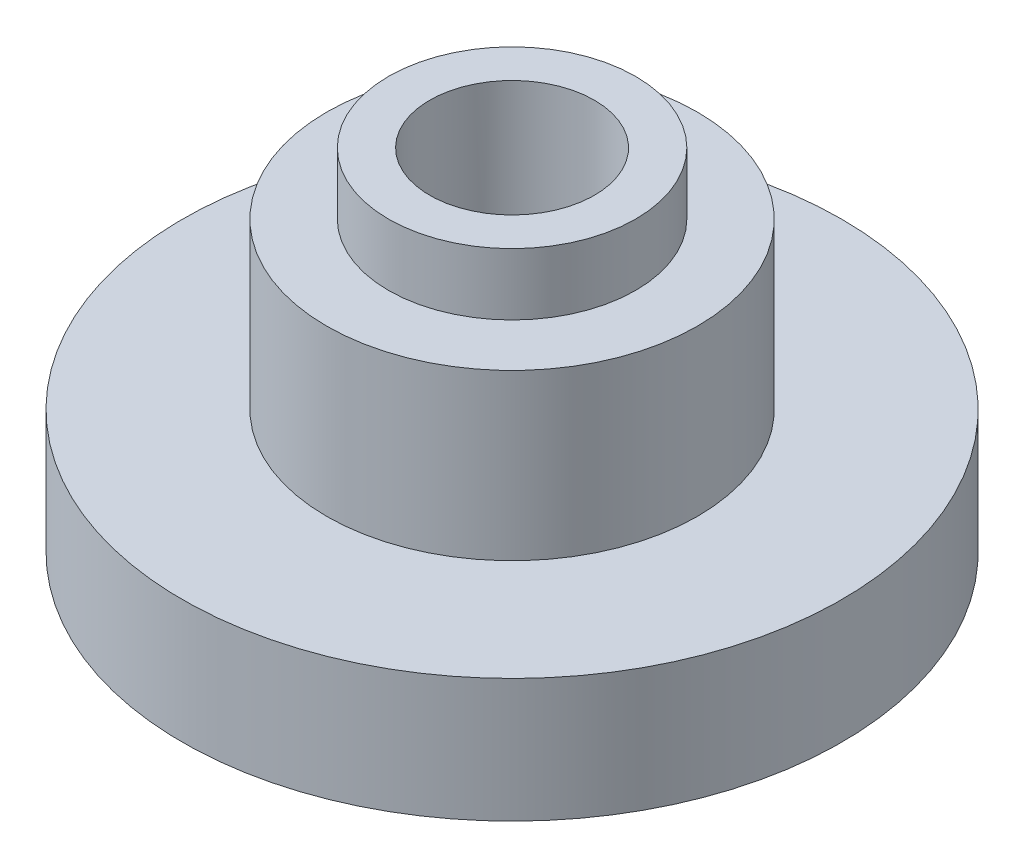
from build123d import *

# Parameters (mm, degrees)
SKETCH_2_R          = 2
CUT_EXTRUDE_1_DEPTH = 10


with BuildPart() as part:
    # 草图1 → 旋转1 (revolve)
    with BuildSketch(Plane.XY, mode=Mode.PRIVATE) as revolve_1_sk:
        Polygon((6, 3.693560261), (6, 0.693560261), (9, 0.693560261), (9, -7.306439739), (16, -7.306439739), (16, -13.306439739), (0, -13.306439739), (0, -9.306439739), (4, -9.306439739), (4, 3.693560261), align=None)
    revolve(revolve_1_sk.sketch.rotate(Axis((0, 0, 0), (0, 1, 0)), 90), axis=Axis((0, 0, 0), (0, 1, 0)))

    # 草图2 → 切除-拉伸1 (cut)
    with BuildSketch(Plane(origin=(0, 0, 0), x_dir=(0, 0, -1), z_dir=(1, 0, 0))):
        with Locations((0, -3.306439739)):
            Circle(SKETCH_2_R)
    extrude(amount=-CUT_EXTRUDE_1_DEPTH, mode=Mode.SUBTRACT)


solid = part.part
